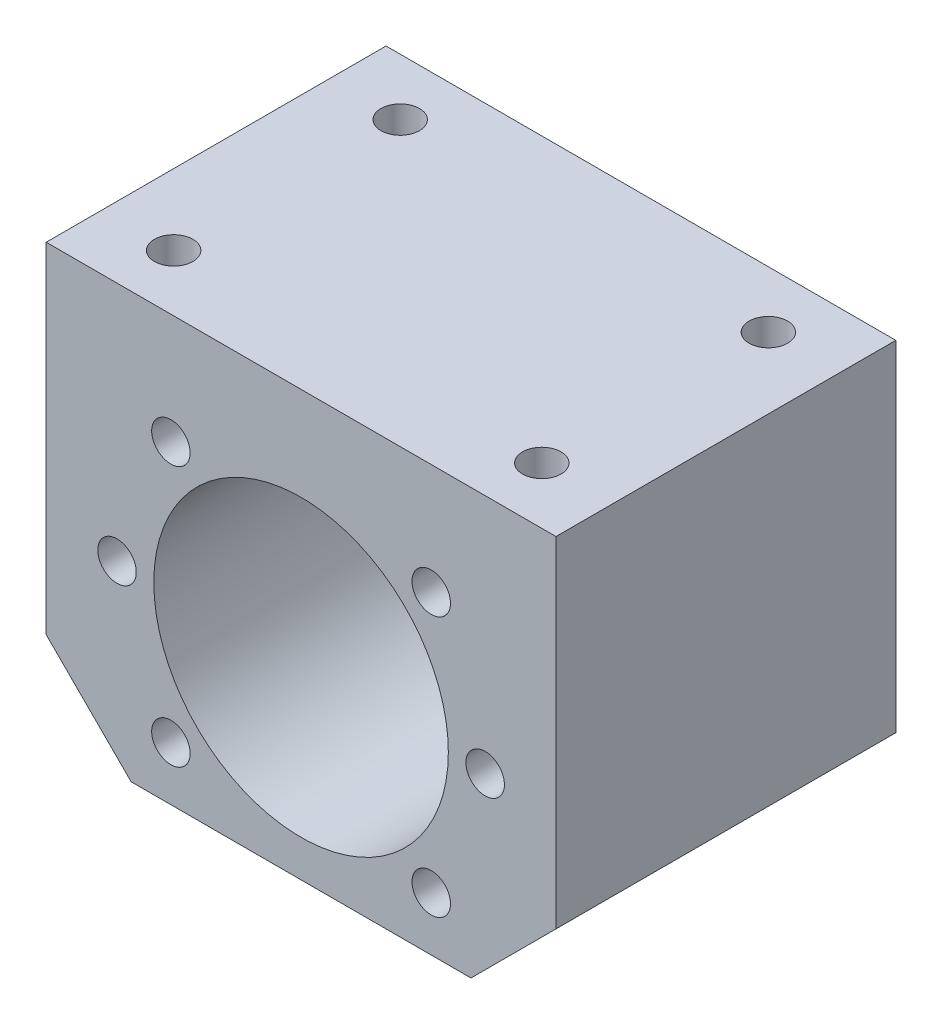
from build123d import *

# Parameters (mm, degrees)
SKETCH_1_W             = 90
SKETCH_1_H             = 75
SKETCH_1_R             = 26
EXTRUDE_1_DEPTH        = 30
HOLE_WIZARD_M8_1_D     = 6.8
HOLE_WIZARD_M8_1_DEPTH = 19.75
HOLE_WIZARD_M8_1_TIP   = 2.042926105
CHAMFER_1_SIZE         = 15
HOLE_WIZARD_M8_2_D     = 6.8
HOLE_WIZARD_M8_2_DEPTH = 19.75
HOLE_WIZARD_M8_2_TIP   = 2.042926105


with BuildPart() as part:
    # 草图1 → 凸台-拉伸1 (new, symmetric)
    with BuildSketch(Plane.XY):
        with Locations((0, 5)):
            Rectangle(SKETCH_1_W, SKETCH_1_H)
        Circle(SKETCH_1_R, mode=Mode.SUBTRACT)
    extrude(amount=EXTRUDE_1_DEPTH, both=True)

    # M8 螺纹孔1
    with Locations(Plane(origin=(-32.5, 0, 30), x_dir=(1, 0, 0), z_dir=(0, 0, 1))):
        with Locations((0, 0), (9.519029611, 22.980970389), (9.519029611, -22.980970389), (55.480970389, -22.980970389), (65, 0), (55.480970389, 22.980970389)):
            Hole(HOLE_WIZARD_M8_1_D / 2, depth=HOLE_WIZARD_M8_1_DEPTH)
            with Locations((0, 0, -(HOLE_WIZARD_M8_1_DEPTH + HOLE_WIZARD_M8_1_TIP / 2))):  # 118° drill point
                Cone(0, HOLE_WIZARD_M8_1_D / 2, HOLE_WIZARD_M8_1_TIP, mode=Mode.SUBTRACT)

    # 倒角1
    chamfer_1_edges = [part.edges().sort_by_distance(p)[0] for p in [
        (45, -32.5, 0),
        (-45, -32.5, 0),
    ]]
    chamfer(chamfer_1_edges, length=CHAMFER_1_SIZE)

    # M8 螺纹孔2
    with Locations(Plane(origin=(32.5, 42.5, -20), x_dir=(1, 0, 0), z_dir=(0, 1, 0))):
        with Locations((0, 0), (0, -40), (-65, -40), (-65, 0)):
            Hole(HOLE_WIZARD_M8_2_D / 2, depth=HOLE_WIZARD_M8_2_DEPTH)
            with Locations((0, 0, -(HOLE_WIZARD_M8_2_DEPTH + HOLE_WIZARD_M8_2_TIP / 2))):  # 118° drill point
                Cone(0, HOLE_WIZARD_M8_2_D / 2, HOLE_WIZARD_M8_2_TIP, mode=Mode.SUBTRACT)


solid = part.part
